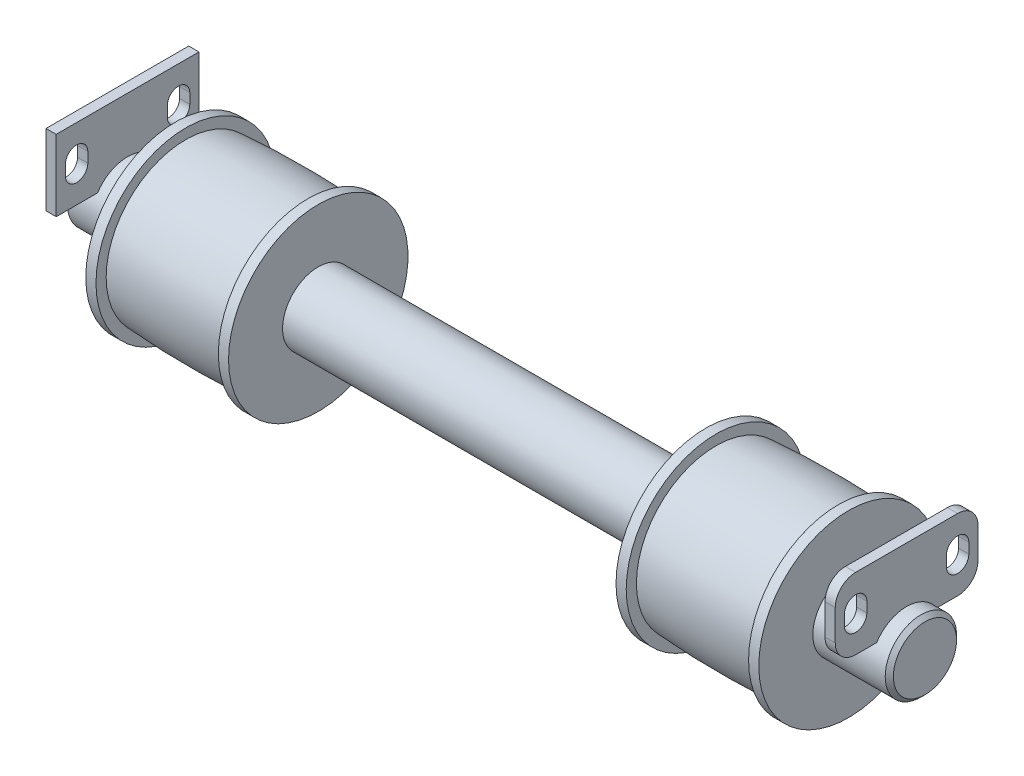
SolidWorks part; units mm, degrees
ref_plane "前视基准面" through (0, 0, 0) normal (0, 0, 1) x (1, 0, 0)
ref_plane "上视基准面" through (0, 0, 0) normal (0, 1, 0) x (1, 0, 0)
ref_plane "右视基准面" through (0, 0, 0) normal (1, 0, 0) x (0, 0, -1)
sketch "草图1" plane through (0, 0, 0) normal (0, 0, 1) x (1, 0, 0)
  line L0 (72263.7407, -3974.1009) -> (72228.2407, -3974.1009)
  line L1 (72158.2407, -3974.1009) -> (71968.2407, -3974.1009)
  line L2 (71898.2407, -3974.1009) -> (71862.7407, -3974.1009)
  line L3 (71860.7407, -3976.1009) -> (71860.7407, -3991.6009)
  line L4 (71862.7407, -3974.1009) -> (71860.7407, -3976.1009)
  line L5 (72263.7407, -3974.1009) -> (72265.7407, -3976.1009)
  line L6 (72265.7407, -3976.1009) -> (72265.7407, -3991.6009)
  line L7 (71898.2407, -3974.1009) -> (71898.2407, -3947.6009)
  line L8 (71898.2407, -3947.6009) -> (71903.2407, -3947.6009)
  line L9 (71963.2407, -3947.6009) -> (71968.2407, -3947.6009)
  line L10 (71968.2407, -3947.6009) -> (71968.2407, -3974.1009)
  line L11 (72223.2407, -3947.6009) -> (72228.2407, -3947.6009)
  line L12 (72228.2407, -3947.6009) -> (72228.2407, -3974.1009)
  line L13 (72223.2407, -3947.6009) -> (72223.2407, -3952.6009)
  line L14 (72163.2407, -3947.6009) -> (72163.2407, -3952.6009)
  line L15 (71963.2407, -3952.6009) -> (71963.2407, -3947.6009)
  line L16 (72163.2407, -3947.6009) -> (72158.2407, -3947.6009)
  line L17 (72158.2407, -3947.6009) -> (72158.2407, -3974.1009)
  line L18 (71860.7407, -3991.6009) -> (72265.7407, -3991.6009) construction
  line L19 (71903.2407, -3947.6009) -> (71903.2407, -3952.6009)
  line L20 (71860.7407, -3991.6009) -> (72265.7407, -3991.6009)
  arc A0 (72223.2407, -3952.6009) -> (72163.2407, -3952.6009) centre (72193.2407, -4402.1009) ccw
  arc A1 (71963.2407, -3952.6009) -> (71903.2407, -3952.6009) centre (71933.2407, -4402.1009) ccw
revolve "旋转1" add sketch "草图1" angle 360 about L18
sketch "草图2" plane through (0, 0, 0) normal (0, 0, 1) x (1, 0, 0)
  line L0 (72265.7407, -4007.1009) -> (72265.7407, -3976.1009) construction
  line L1 (72251.7407, -3982.1009) -> (72256.7407, -3982.1009)
  line L2 (72251.7407, -3982.1009) -> (72251.7407, -3956.3341)
  line L3 (72251.7407, -3956.3341) -> (72256.7407, -3956.3341)
  line L4 (72256.7407, -3982.1009) -> (72256.7407, -3956.3341)
  line L5 (72263.7407, -3974.1009) -> (72228.2407, -3974.1009) construction
  line L6 (72063.2407, -3974.1009) -> (72063.2407, -3913.7867) construction
  line L7 (72158.2407, -3974.1009) -> (71968.2407, -3974.1009) construction
  line L8 (71869.7407, -3982.1009) -> (71869.7407, -3956.3341)
  line L9 (71874.7407, -3956.3341) -> (71869.7407, -3956.3341)
  line L10 (71874.7407, -3982.1009) -> (71874.7407, -3956.3341)
  line L11 (71874.7407, -3982.1009) -> (71869.7407, -3982.1009)
  dimension "D1" = 9
  dimension "D2" = 8
  dimension "D3" = 5
extrude "切除-拉伸1" cut sketch "草图2" against normal through all both and the other way through all
sketch "草图3" plane through (0, -3982.1009, 0) normal (0, 1, 0) x (1, 0, 0)
  line L0 (72251.7407, -14.6969) -> (72251.7407, 14.6969) construction
  line L1 (72251.7407, 35) -> (72256.7407, 35)
  line L2 (72251.7407, 35) -> (72251.7407, -35)
  line L3 (72251.7407, -35) -> (72256.7407, -35)
  line L4 (72256.7407, 35) -> (72256.7407, -35)
  line L5 (72256.7407, 14.6969) -> (72256.7407, -14.6969) construction
  line L6 (72256.7407, 0) -> (72291.1005, 0) construction
  line L7 (72063.2407, 17.5) -> (72063.2407, 72.9517) construction
  line L8 (72158.2407, 17.5) -> (71968.2407, 17.5) construction
  line L9 (71869.7407, 35) -> (71869.7407, -35)
  line L10 (71874.7407, -35) -> (71869.7407, -35)
  line L11 (71874.7407, 35) -> (71874.7407, -35)
  line L12 (71874.7407, 35) -> (71869.7407, 35)
  dimension "D1" = 70
extrude "凸台-拉伸1" add sketch "草图3" along normal blind 35 separate body
fillet "圆角1" radius 10 4 edges at (72254.2407, -3982.1009, 35) (72254.2407, -3947.1009, 35) (72254.2407, -3982.1009, -35) (72254.2407, -3947.1009, -35)
sketch "草图4" plane through (72256.7407, 0, 0) normal (1, 0, 0) x (0, 0, -1)
  line L0 (-35, -3964.6009) -> (35, -3964.6009) construction
  line L1 (-35, -3957.1009) -> (-35, -3972.1009) construction
  line L2 (35, -3957.1009) -> (35, -3972.1009) construction
  line L3 (0, -3964.6009) -> (0, -3952.2034) construction
  line L4 (-25, -3962.1009) -> (-25, -3967.1009) construction
  line L7 (-19.5, -3962.1009) -> (-19.5, -3967.1009)
  line L10 (-30.5, -3962.1009) -> (-30.5, -3967.1009)
  line L11 (25, -3962.1009) -> (25, -3967.1009) construction
  line L12 (19.5, -3962.1009) -> (19.5, -3967.1009)
  line L13 (30.5, -3962.1009) -> (30.5, -3967.1009)
  arc A6 (-19.5, -3962.1009) -> (-30.5, -3962.1009) centre (-25, -3962.1009) ccw
  arc A7 (-30.5, -3967.1009) -> (-19.5, -3967.1009) centre (-25, -3967.1009) ccw
  arc A8 (19.5, -3962.1009) -> (30.5, -3962.1009) centre (25, -3962.1009) cw
  arc A9 (30.5, -3967.1009) -> (19.5, -3967.1009) centre (25, -3967.1009) cw
  point P8 (-25, -3964.6009)
  point P18 (25, -3964.6009)
  dimension "D1" = 5.5
  dimension "D2" = 16
  dimension "D3" = 50
extrude "切除-拉伸2" cut sketch "草图4" against normal through all both and the other way through all contours A9 L12 A8 L13
